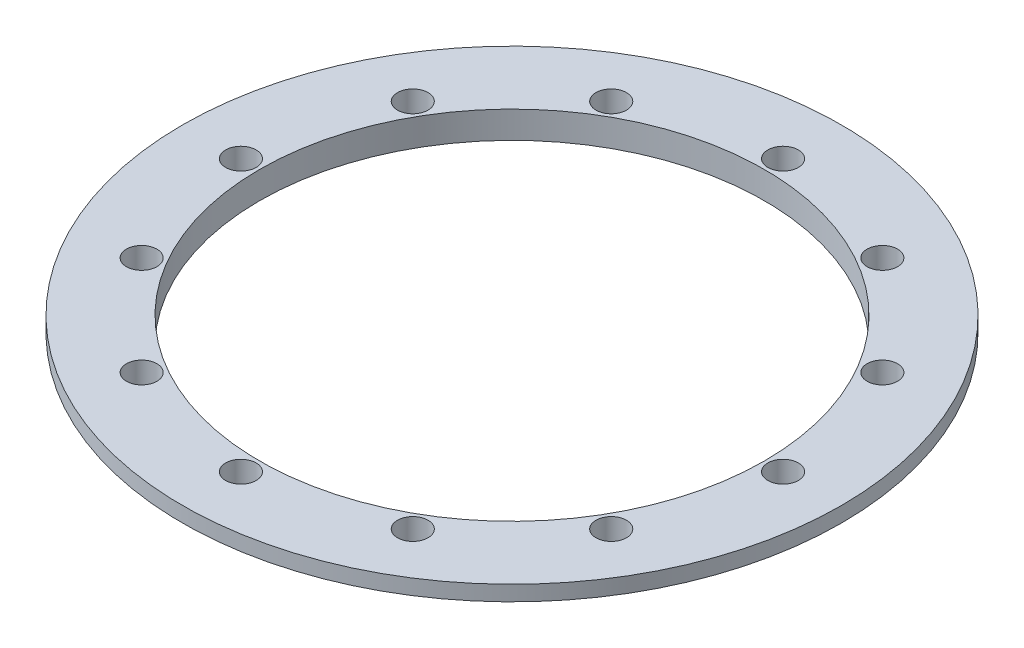
from build123d import *

# Parameters (mm, degrees)
FILLET1_R                                            = 1.6
HOLE_SIZE_PER_SOCKET_HEAD_CAP_SCREW_TYPE_D           = 11
HOLE_SIZE_PER_SOCKET_HEAD_CAP_SCREW_TYPE_CBORE_D     = 18
HOLE_SIZE_PER_SOCKET_HEAD_CAP_SCREW_TYPE_CBORE_DEPTH = 13
CIRPATTERN1_COUNT                                    = 12


with BuildPart() as part:
    # Sketch1 → Revolve1 (revolve)
    with BuildSketch(Plane.XY):
        Polygon((-149, 0), (-149, 16), (-194.5, 16), (-194.5, 7), (-177, 7), (-177, 0), align=None)
    revolve(axis=Axis((0, 32.824838348, 0), (0, -1, 0)))

    # Fillet1
    fillet1_edges = [part.edges().sort_by_distance(p)[0] for p in [
        (177, 7, 0),
    ]]
    fillet(fillet1_edges, radius=FILLET1_R)

    # Hole size per socket head cap screw type1 (through all)
    with Locations(Plane(origin=(0, 16, 0), x_dir=(-1, 0, 0), z_dir=(0, 1, 0))):
        with Locations((160, 0)):
            hole_size_per_socket_head_cap_screw_type = CounterBoreHole(HOLE_SIZE_PER_SOCKET_HEAD_CAP_SCREW_TYPE_D / 2, HOLE_SIZE_PER_SOCKET_HEAD_CAP_SCREW_TYPE_CBORE_D / 2, HOLE_SIZE_PER_SOCKET_HEAD_CAP_SCREW_TYPE_CBORE_DEPTH)

    # CirPattern1: Hole size per socket head cap screw type1 ×12 about axis
    cirpattern1_axis = Axis((0, 0, 0), (0, 1, 0))
    for i in range(1, CIRPATTERN1_COUNT):
        add(hole_size_per_socket_head_cap_screw_type.rotate(cirpattern1_axis, i * 360 / CIRPATTERN1_COUNT), mode=Mode.SUBTRACT)


solid = part.part
